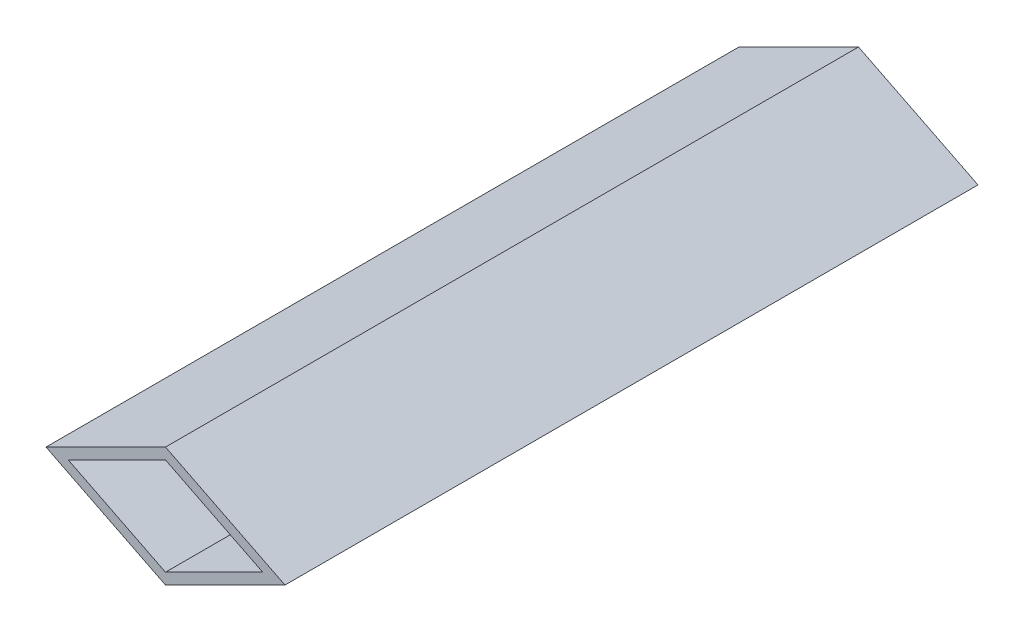
SolidWorks part; units mm, degrees
ref_plane "Front Plane" through (0, 0, 0) normal (0, 0, 1) x (1, 0, 0)
ref_plane "Top Plane" through (0, 0, 0) normal (0, 1, 0) x (1, 0, 0)
ref_plane "Right Plane" through (0, 0, 0) normal (1, 0, 0) x (0, 0, -1)
sketch "Sketch1" plane through (0, 0, 0) normal (0, 0, 1) x (1, 0, 0)
  line L0 (0, 169.9115) -> (-60, 139.9115) construction
  line L1 (-60, 139.9115) -> (0, 109.9115) construction
  line L2 (0, 109.9115) -> (60, 139.9115) construction
  line L3 (60, 139.9115) -> (0, 169.9115) construction
  line L4 (0, 169.9115) -> (-60, 139.9115)
  line L5 (-60, 139.9115) -> (0, 109.9115)
  line L6 (0, 109.9115) -> (60, 139.9115)
  line L7 (60, 139.9115) -> (0, 169.9115)
extrude "Boss-Extrude1" add sketch "Sketch1" along normal blind 348
sketch "Sketch2" plane through (0, 0, 348) normal (0, 0, 1) x (1, 0, 0)
  line L8 (48.8197, 139.9115) -> (0, 164.3214)
  line L9 (0, 164.3214) -> (-48.8197, 139.9115)
  line L10 (-48.8197, 139.9115) -> (0, 115.5017)
  line L11 (0, 115.5017) -> (48.8197, 139.9115)
  line L12 (48.8197, 139.9115) -> (0, 164.3214)
  line L13 (0, 164.3214) -> (-48.8197, 139.9115)
  line L14 (-48.8197, 139.9115) -> (0, 115.5017)
  line L15 (0, 115.5017) -> (48.8197, 139.9115)
  dimension "D1" = 5
extrude "Cut-Extrude1" cut sketch "Sketch2" against normal blind 350
